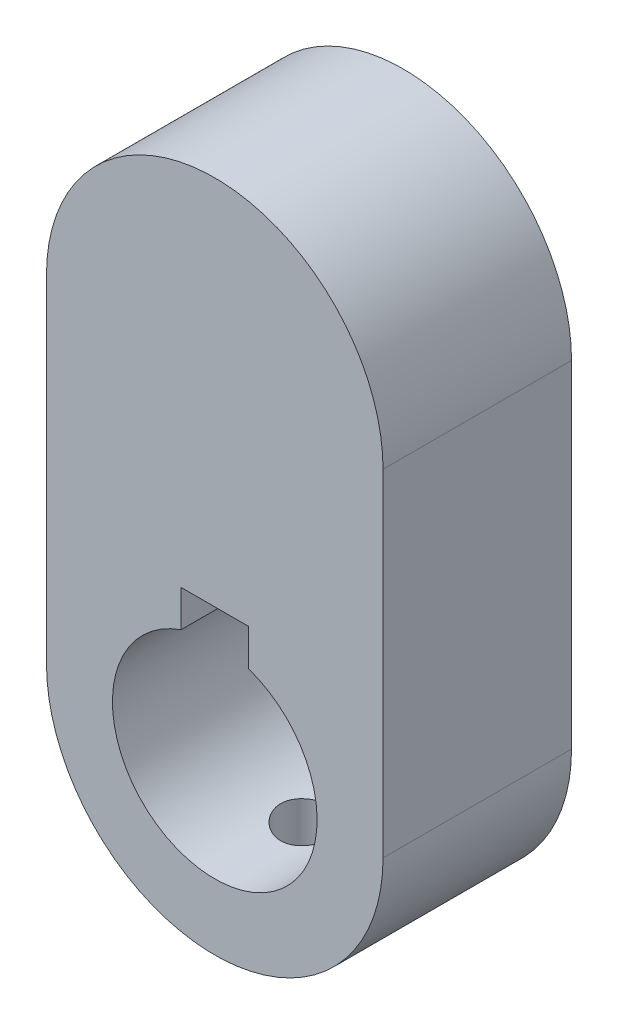
SolidWorks part; units mm, degrees
material "Q235B"
ref_plane "Front Plane" through (0, 0, 0) normal (0, 0, 1) x (1, 0, 0)
ref_plane "Top Plane" through (0, 0, 0) normal (0, 1, 0) x (1, 0, 0)
ref_plane "Right Plane" through (0, 0, 0) normal (1, 0, 0) x (0, 0, -1)
sketch "Sketch1" plane through (0, 0, 0) normal (0, 0, 1) x (1, 0, 0)
  line L0 (0, 0) -> (0, 25) construction
  line L1 (-12.5, 0) -> (-12.5, 25)
  line L2 (12.5, 0) -> (12.5, 25)
  line L4 (2.5, 5.3) -> (-2.5, 5.3)
  line L5 (2.5, 5.3) -> (2.5, 9.9)
  line L6 (2.5, 9.9) -> (-2.5, 9.9)
  line L7 (-2.5, 5.3) -> (-2.5, 9.9)
  line L8 (2.5, 5.3) -> (-2.5, 9.9) construction
  line L9 (2.5, 9.9) -> (-2.5, 5.3) construction
  arc A0 (-12.5, 0) -> (12.5, 0) centre (0, 0) ccw
  arc A1 (12.5, 25) -> (-12.5, 25) centre (0, 25) ccw
  circle A2 centre (0, 0) radius 7.6
  point P3 (0, 12.5)
  point P10 (0, 7.6)
  dimension "D2" = 12.5
  dimension "D3" = 15.2
  dimension "D4" = 5
  dimension "D1" = 25
  dimension "D5" = 17.5
extrude "Boss-Extrude1" add sketch "Sketch1" along normal blind 14 contours L2 A1 L1 A0 A2 L7 L6 L5
hole_wizard "M5 Tapped Hole1" positions "Sketch2" profile "Sketch3" tap size "M5" standard "GB"
sketch "Sketch2" plane through (0, 0, 0) normal (0, 1, 0) x (1, 0, 0)
  line L0 (12.5, 0) -> (-12.5, 0) construction
  point P0 (0, -7)
  dimension "D1" = 7
sketch "Sketch3" plane through (0, 0, 7) normal (1, 0, 0) x (0, 0, 1)
  line L0 (0, 0) -> (0, 12.5)
  line L1 (0, 12.5) -> (2.1, 12.5)
  line L2 (2.1, 12.5) -> (2.1, 0)
  line L5 (2.1, 0) -> (0, 0)
  line L11 (0, -6.35) -> (0, 107.95) construction
  dimension "通孔螺纹孔钻头直径" = 4.2
  dimension "通孔螺纹孔钻头深度" = 12.5
cosmetic thread "Hole Thread1" parameters "D2"=5
